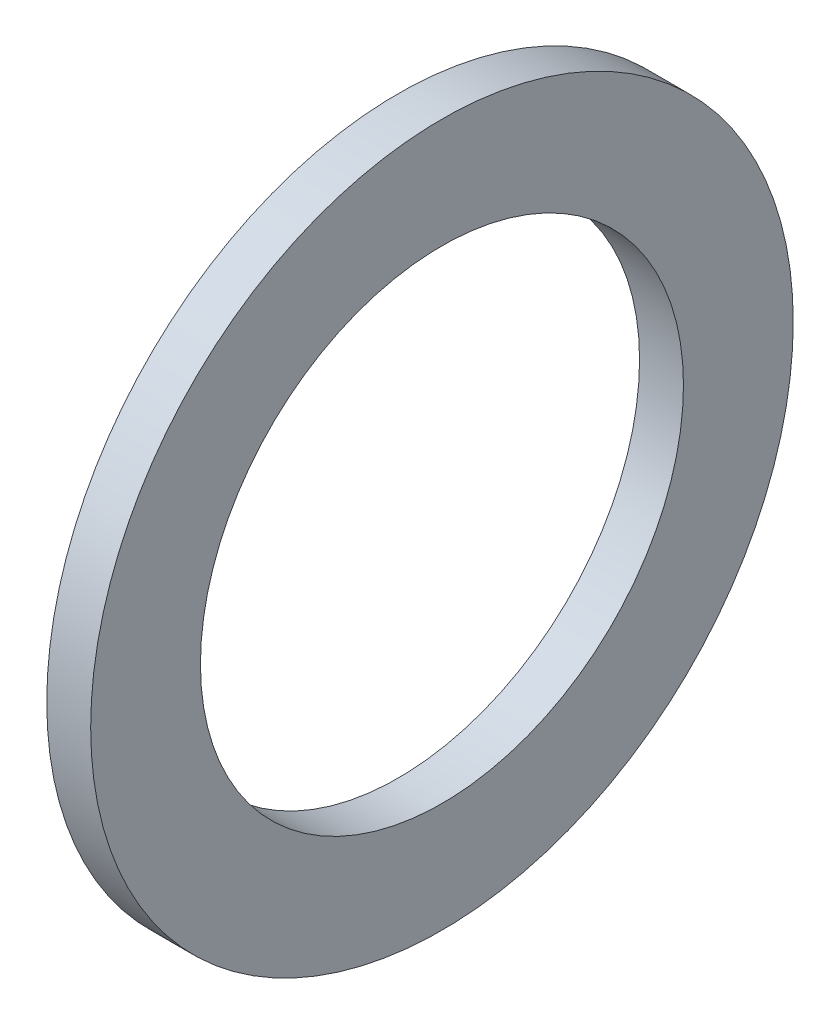
from build123d import *

# Parameters (mm, degrees)
SKETCH1_W = 2
SKETCH1_H = 5


with BuildPart() as part:
    # Sketch1 → Revolve1 (revolve)
    with BuildSketch(Plane.XY, mode=Mode.PRIVATE) as revolve1_sk:
        with Locations((1, 13.5)):
            Rectangle(SKETCH1_W, SKETCH1_H)
    revolve(revolve1_sk.sketch.rotate(Axis((0, 0, 0), (-1, 0, 0)), 90), axis=Axis((0, 0, 0), (-1, 0, 0)))


solid = part.part
